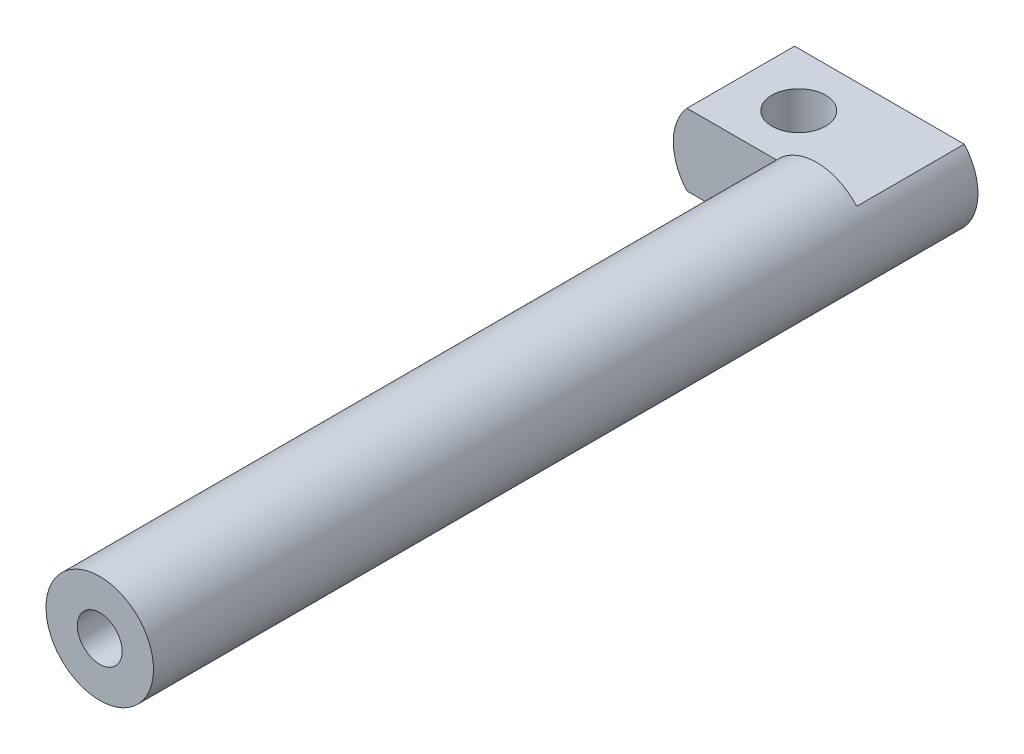
from build123d import *
from build123d.topology import SkipClean

# Parameters (mm, degrees)
SKETCH1_R           = 3
SKETCH1_R_2         = 1.25
BOSS_EXTRUDE1_DEPTH = 40
BOSS_EXTRUDE2_START = 6
SKETCH2_R           = 1.25
BOSS_EXTRUDE2_DEPTH = 6
SKETCH3_W           = 27.527522068
SKETCH3_H           = 18.672368854
SKETCH3_W_2         = 16.126466482
SKETCH3_H_2         = 4
CUT_EXTRUDE1_DEPTH  = 6
SKETCH4_R           = 1.5
CUT_EXTRUDE2_DEPTH  = 16


with BuildPart() as part:
    # Sketch1 → Boss-Extrude1 (new body)
    with BuildSketch(Plane.XY):
        Circle(SKETCH1_R)
        Circle(SKETCH1_R_2, mode=Mode.SUBTRACT)
    extrude(amount=BOSS_EXTRUDE1_DEPTH)

    # Sketch2 → Boss-Extrude2 (add)
    with SkipClean():  # the faces are left unmerged after this step: merging them gives an invalid solid
        with BuildSketch(Plane(origin=(0, 0, 0), x_dir=(-1, 0, 0), z_dir=(0, 0, -1)).offset(BOSS_EXTRUDE2_START)):
            with BuildLine():
                Line((0, 3), (5, 3))
                ThreePointArc((5, 3), (8, 0), (5, -3))
                Line((5, -3), (0, -3))
                ThreePointArc((0, -3), (-3, 0), (0, 3))
            make_face()
            Circle(SKETCH2_R, mode=Mode.SUBTRACT)
        extrude(amount=-BOSS_EXTRUDE2_DEPTH)

    # Sketch3 → Cut-Extrude1 (cut)
    with SkipClean():  # the faces are left unmerged after this step: merging them gives an invalid solid
        with BuildSketch(Plane(origin=(0, 0, -6), x_dir=(-1, 0, 0), z_dir=(0, 0, -1))):
            with Locations((1.25, 0)):
                Rectangle(SKETCH3_W, SKETCH3_H)
            with Locations((1.25, 0)):
                Rectangle(SKETCH3_W_2, SKETCH3_H_2, mode=Mode.SUBTRACT)
        extrude(amount=-CUT_EXTRUDE1_DEPTH, mode=Mode.SUBTRACT)

    # Sketch4 → Cut-Extrude2 (cut)
    with SkipClean():  # the faces are left unmerged after this step: merging them gives an invalid solid
        with BuildSketch(Plane(origin=(0, -2, 0), x_dir=(-1, 0, 0), z_dir=(0, -1, 0))):
            with Locations(Location((4, 3, 0), (0, 0, 90))):
                Circle(SKETCH4_R)
        extrude(amount=-CUT_EXTRUDE2_DEPTH, mode=Mode.SUBTRACT)


solid = part.part
